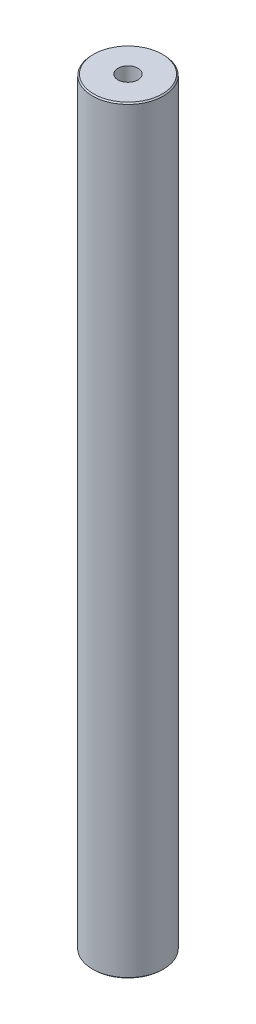
SolidWorks part; units mm, degrees
material "Q235A"
ref_plane "前基準面" through (0, 0, 0) normal (0, 0, 1) x (1, 0, 0)
ref_plane "上基準面" through (0, 0, 0) normal (0, 1, 0) x (1, 0, 0)
ref_plane "右基準面" through (0, 0, 0) normal (1, 0, 0) x (0, 0, -1)
sketch "草图1" plane through (0, 0, 0) normal (0, 1, 0) x (1, 0, 0)
  circle A0 centre (0, 0) radius 15
  dimension "D1" = 30
extrude "凸台-拉伸1" add sketch "草图1" along normal mid plane 320
chamfer "倒角1" distance 0.5 angle 45 2 edges at (0, -160, 15) (0, 160, 15)
hole_wizard "M10 螺纹孔2" positions "草图2" profile "草图3" tap size "M10" standard "GB"
sketch "草图2" plane through (0, 160, 0) normal (0, 1, 0) x (1, 0, 0)
  point P0 (0, 0)
sketch "草图3" plane through (0, 160, 0) normal (1, 0, 0) x (0, 0, 1)
  line L0 (0, 0) -> (0, 27.0537)
  line L1 (0, 27.0537) -> (4.25, 24.5)
  line L2 (4.25, 24.5) -> (4.25, 0)
  line L5 (4.25, 0) -> (0, 0)
  line L10 (0, 27.0537) -> (-4.25, 24.5) construction
  line L11 (0, -6.35) -> (0, 107.95) construction
  dimension "螺纹孔钻头直径" = 8.5
  dimension "螺纹孔钻头深度" = 24.5
  dimension "导头角度" = 118
cosmetic thread "孔螺蚊线1" parameters "D1"=20, "D2"=10
hole_wizard "M10 螺纹孔1" positions "草图4" profile "草图5" tap size "M10" standard "GB"
sketch "草图4" plane through (0, -160, 0) normal (0, -1, 0) x (-1, 0, 0)
  point P0 (0, 0)
sketch "草图5" plane through (0, -160, 0) normal (1, 0, 0) x (0, 0, -1)
  line L0 (0, 0) -> (0, 27.0537)
  line L1 (0, 27.0537) -> (4.25, 24.5)
  line L2 (4.25, 24.5) -> (4.25, 0)
  line L5 (4.25, 0) -> (0, 0)
  line L10 (0, 27.0537) -> (-4.25, 24.5) construction
  line L11 (0, -6.35) -> (0, 107.95) construction
  dimension "螺纹孔钻头直径" = 8.5
  dimension "螺纹孔钻头深度" = 24.5
  dimension "导头角度" = 118
cosmetic thread "孔螺蚊线2" parameters "D1"=20, "D2"=10
